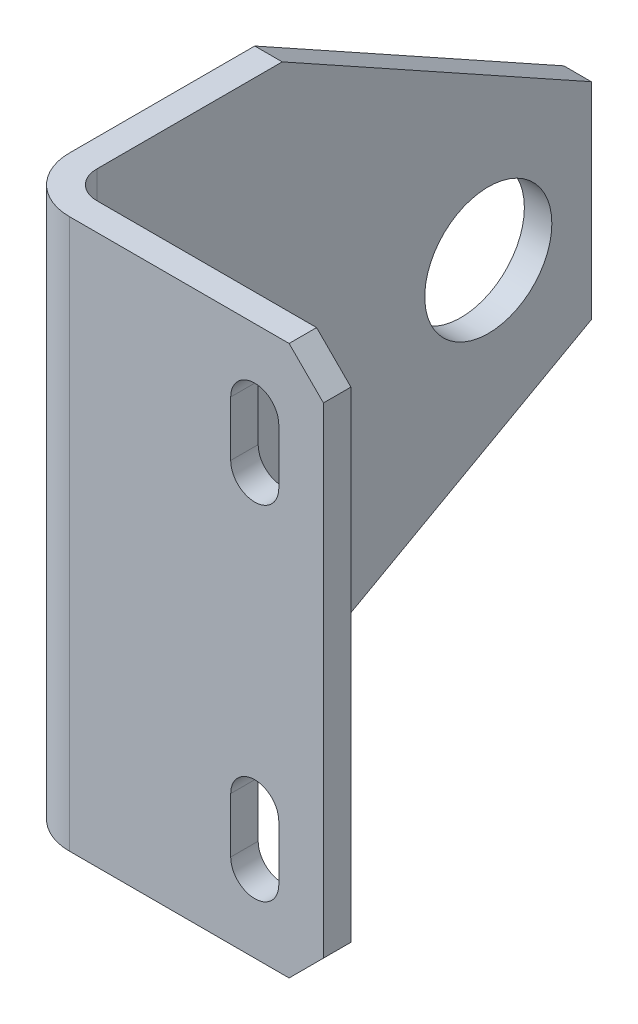
SolidWorks part; units mm, degrees
material "1023 碳钢板 (SS)"
ref_plane "前视基准面" through (0, 0, 0) normal (0, 0, 1) x (1, 0, 0)
ref_plane "上视基准面" through (0, 0, 0) normal (0, 1, 0) x (1, 0, 0)
ref_plane "右视基准面" through (0, 0, 0) normal (1, 0, 0) x (0, 0, -1)
sketch "草图1" plane through (0, 0, 0) normal (1, 0, 0) x (0, 0, -1)
  line L0 (-45, 0) -> (27, 40)
  line L1 (27, 40) -> (-45, 80)
  line L2 (-45, 80) -> (-80, 80)
  line L3 (-80, 80) -> (-80, 0)
  line L4 (-80, 0) -> (-45, 0)
extrude "凸台-拉伸1" add sketch "草图1" against normal blind 4
sketch "草图2" plane through (0, 0, 0) normal (1, 0, 0) x (0, 0, -1)
  line L0 (-80, 0) -> (-80, 80)
  line L1 (-80, 80) -> (-76, 80)
  line L2 (-76, 80) -> (-76, 0)
  line L3 (-76, 0) -> (-80, 0)
extrude "凸台-拉伸2" add sketch "草图2" along normal blind 41
sketch "草图3" plane through (0, 0, 80) normal (0, 0, 1) x (1, 0, 0)
  line L0 (34.5, 61) -> (34.5, 69)
  line L1 (27.5, 69) -> (27.5, 61)
  arc A0 (27.5, 61) -> (34.5, 61) centre (31, 61) ccw
  arc A1 (34.5, 69) -> (27.5, 69) centre (31, 69) ccw
extrude "切除-拉伸1" cut sketch "草图3" against normal through all
sketch "草图4" plane through (0, 0, 76) normal (0, 0, -1) x (-1, 0, 0)
  line L0 (-34.5, 19) -> (-34.5, 11)
  line L1 (-27.5, 11) -> (-27.5, 19)
  arc A0 (-27.5, 19) -> (-34.5, 19) centre (-31, 19) ccw
  arc A1 (-34.5, 11) -> (-27.5, 11) centre (-31, 11) ccw
extrude "切除-拉伸2" cut sketch "草图4" against normal through all
hole_wizard "Ø18.5 (18.5) 直径孔1" positions "草图6" profile "草图5" hole size "Ø18.5" standard "ANSI Metric"
sketch "草图6" plane through (0, 0, 0) normal (1, 0, 0) x (0, 0, -1)
  point P0 (-15, 40)
sketch "草图5" plane through (0, 40, 15) normal (0, 1, 0) x (0, 0, -1)
  line L0 (0, 0) -> (0, 4)
  line L1 (0, 4) -> (9.25, 4)
  line L2 (9.25, 4) -> (9.25, 0)
  line L5 (9.25, 0) -> (0, 0)
  line L11 (0, -6.35) -> (0, 107.95) construction
  dimension "通孔孔直径" = 18.5
  dimension "通孔孔深度" = 4
chamfer "倒角1" distance 5 angle 45 2 edges at (41, 0, 78) (41, 80, 78)
chamfer "倒角2" distance 30.8869 angle 60.945 1 edges at (-2, 40, -27)
fillet "圆角1" radius 4 1 edges at (0, 40, 76)
fillet "圆角2" radius 8 1 edges at (-4, 40, 80)
